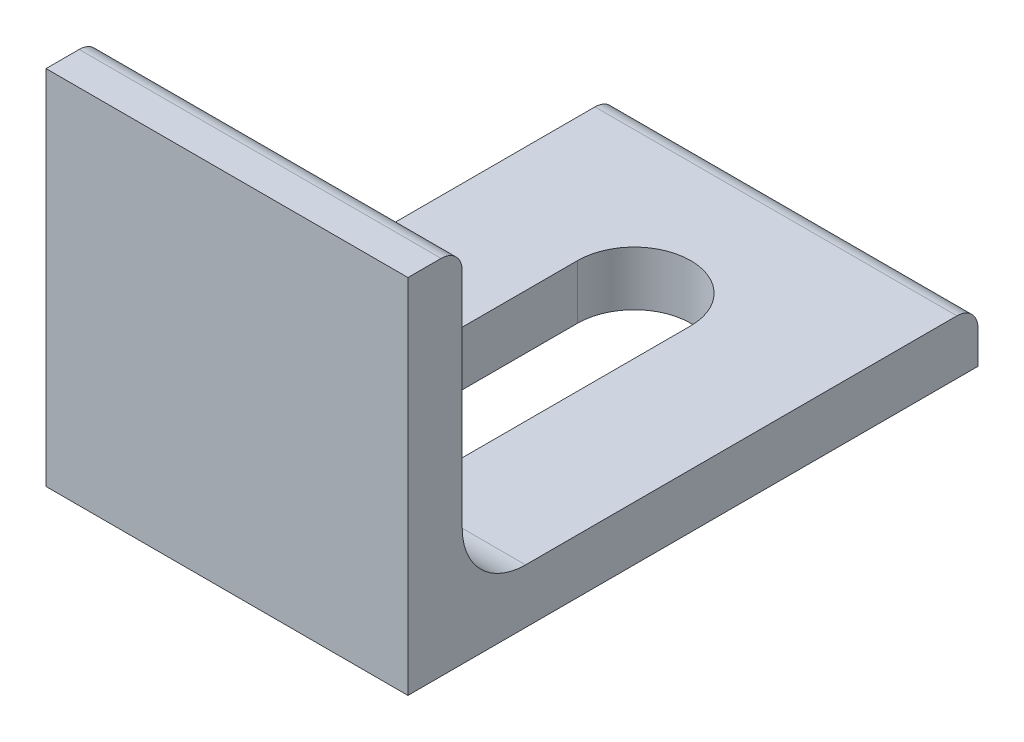
SolidWorks part; units mm, degrees
material "普通碳钢"
ref_plane "前视基准面" through (0, 0, 0) normal (0, 0, 1) x (1, 0, 0)
ref_plane "上视基准面" through (0, 0, 0) normal (0, 1, 0) x (1, 0, 0)
ref_plane "右视基准面" through (0, 0, 0) normal (1, 0, 0) x (0, 0, -1)
sketch3d "3D草图1"
  line L0 (220, 114, 0) -> (180, 114, 0)
  line L1 (245, 114, 0) -> (285, 114, 0) construction
  dimension "D1" = 40
other "热轧不等边角钢gb∕t706-2008 63 X 40 X 6(1)"
ref_plane "基准面1" through (220, 114, 0) normal (-1, 0, 0) x (0, 1, 0)
sketch "Sketch1" plane through (220, 114, 0) normal (-1, 0, 0) x (0, 1, 0)
  line L0 (0, 0) -> (0, 63)
  line L1 (0, 31.5) -> (6, 31.5) construction
  line L2 (6, 60.6667) -> (6, 13)
  line L3 (13, 6) -> (37.6667, 6)
  line L4 (20, 6) -> (20, 0) construction
  line L5 (40, 0) -> (0, 0)
  line L6 (0, 63) -> (3.6667, 63)
  line L7 (40, 0) -> (40, 3.6667)
  arc A0 (40, 3.6667) -> (37.6667, 6) centre (37.6667, 3.6667) ccw
  arc A1 (3.6667, 63) -> (6, 60.6667) centre (3.6667, 60.6667) cw
  arc A2 (13, 6) -> (6, 13) centre (13, 13) cw
  point P10 (20, 0)
  point P14 (0, 31.5)
  point P15 (6, 31.5)
  point P16 (20, 6)
  point P21 (0, 0)
sketch "草图2" plane through (0, 120, 0) normal (0, 1, 0) x (1, 0, 0)
  line L0 (200, 45) -> (200, 20) construction
  line L1 (206.25, 45) -> (206.25, 20)
  line L2 (193.75, 45) -> (193.75, 20)
  line L3 (180, 13) -> (180, 60.6667) construction
  line L4 (220, 0) -> (180, 0) construction
  arc A0 (206.25, 45) -> (193.75, 45) centre (200, 45) ccw
  arc A1 (193.75, 20) -> (206.25, 20) centre (200, 20) ccw
  point P2 (200, 32.5)
  dimension "D1" = 12.5
  dimension "D2" = 25
  dimension "D3" = 20
  dimension "D4" = 20
extrude "切除-拉伸1" cut sketch "草图2" against normal blind 10
equation "\"D2@Sketch1\" = \"Radius_1@Sketch1\" / 3"
equation "\"D4@Sketch1\" = \"D1@Sketch1\""
